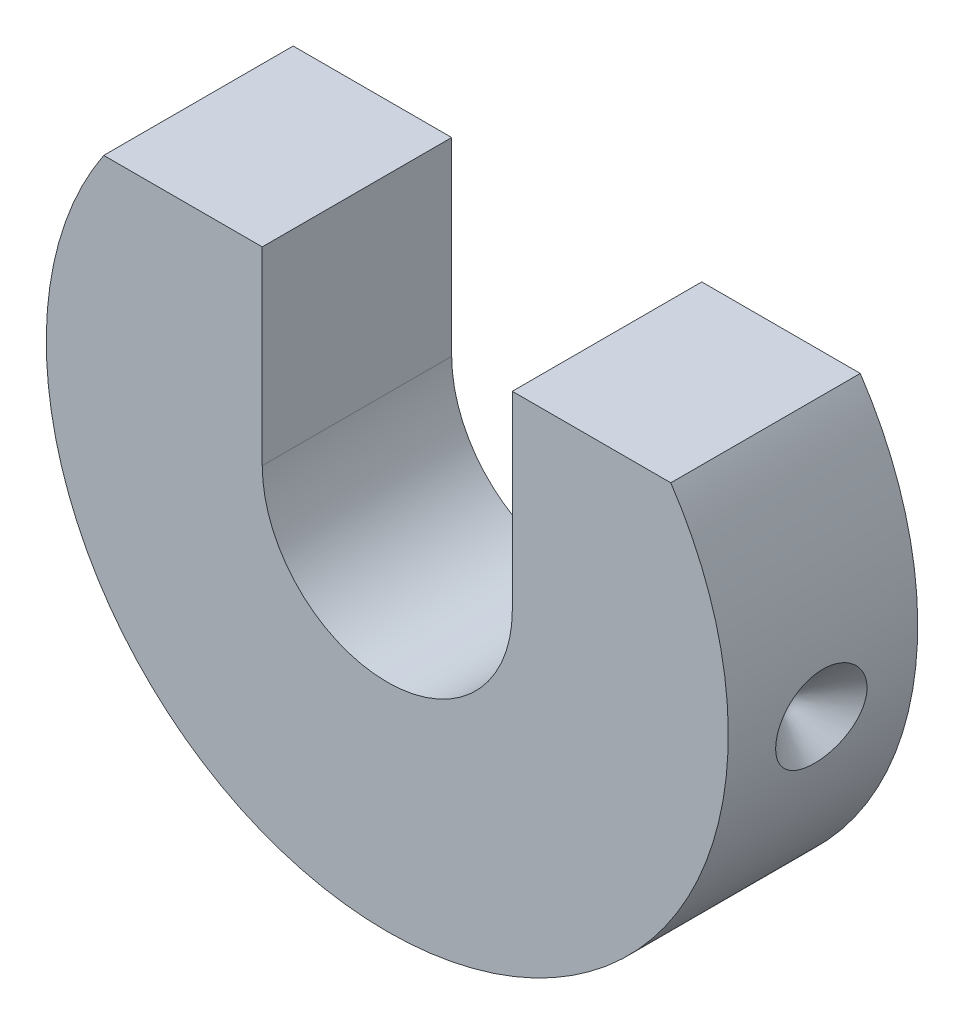
from build123d import *

# Parameters (mm, degrees)
BOSS_EXTRUDE1_DEPTH = 5


with BuildPart() as part:
    # Sketch1 → Boss-Extrude1 (new, symmetric)
    with BuildSketch(Plane.XY):
        with BuildLine():
            Line((-14.966629547, 10), (-6.6, 10))
            Line((-6.6, 10), (-6.6, 0))
            ThreePointArc((-6.6, 0), (0, -6.6), (6.6, 0))
            Line((6.6, 0), (6.6, 10))
            Line((6.6, 10), (14.966629547, 10))
            ThreePointArc((14.966629547, 10), (0, -18), (-14.966629547, 10))
        make_face()
    extrude(amount=BOSS_EXTRUDE1_DEPTH, both=True)

    # Sketch2 → Cut-Revolve1 (revolve, cut)
    with BuildSketch(Plane.XY, mode=Mode.PRIVATE) as cut_revolve1_sk:
        Polygon((18.861572054, -5.361572054), (18.861572054, -2), (15.5, -2), align=None)
    cut_revolve1 = revolve(cut_revolve1_sk.sketch.rotate(Axis((-24.047626866, -2, 0), (1, 0, 0)), 90), axis=Axis((-24.047626866, -2, 0), (1, 0, 0)), mode=Mode.SUBTRACT)

    # Mirror1: Cut-Revolve1 across plane
    add(cut_revolve1.mirror(Plane(origin=(0, 0, 0), x_dir=(0, 0, 1), z_dir=(1, 0, 0))), mode=Mode.SUBTRACT)


solid = part.part
